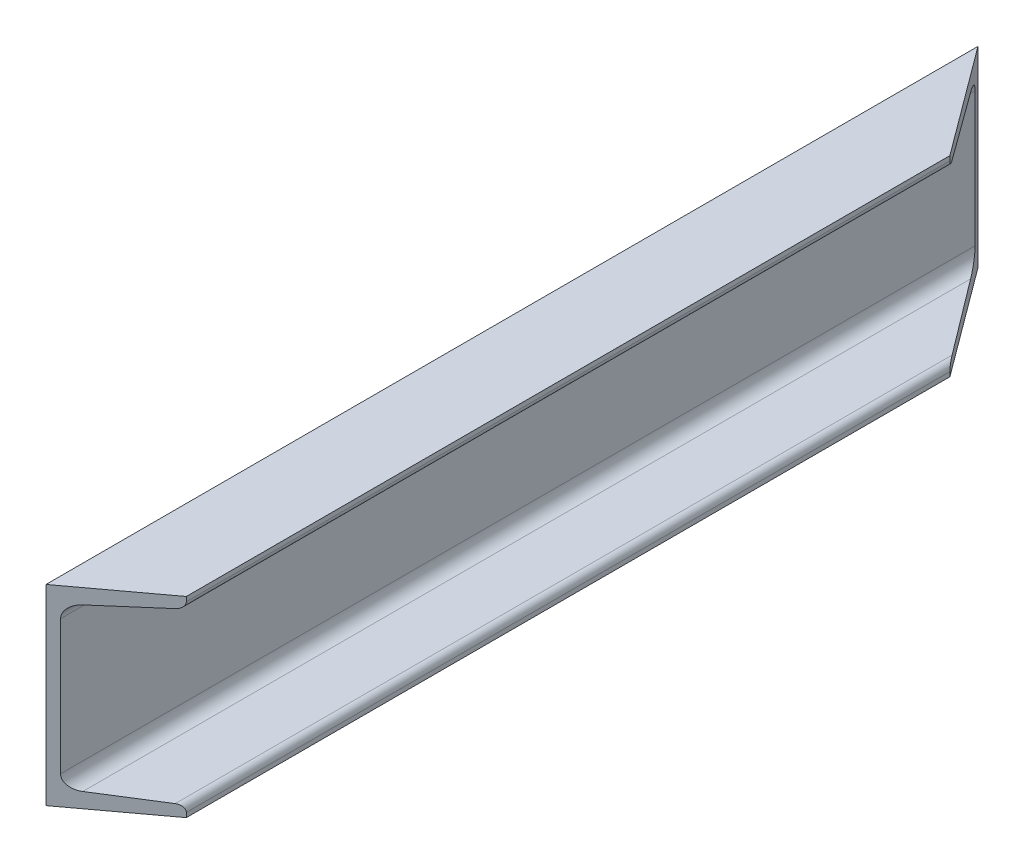
SolidWorks part; units mm, degrees
material "普通碳钢"
ref_plane "Front Plane" through (0, 0, 0) normal (0, 0, 1) x (1, 0, 0)
ref_plane "Top Plane" through (0, 0, 0) normal (0, 1, 0) x (1, 0, 0)
ref_plane "Right Plane" through (0, 0, 0) normal (1, 0, 0) x (0, 0, -1)
sketch "Sketch1" plane through (0, 0, 0) normal (0, 0, 1) x (1, 0, 0)
  line L0 (0, 63) -> (0, -63)
  line L1 (-28.7334, 0) -> (89.5233, 0) construction
  line L2 (0, 63) -> (53, 63)
  line L3 (53, 63) -> (53, 60.0159)
  line L4 (48.8069, 55.5264) -> (13.8863, 53.1396)
  line L5 (5.5, 44.1606) -> (5.5, -44.1606)
  line L6 (0, -63) -> (53, -63)
  line L7 (53, -63) -> (53, -60.0159)
  line L8 (48.8069, -55.5264) -> (13.8863, -53.1396)
  arc A0 (53, 60.0159) -> (48.8069, 55.5264) centre (48.5, 60.0159) cw
  arc A1 (13.8863, 53.1396) -> (5.5, 44.1606) centre (14.5, 44.1606) ccw
  arc A2 (13.8863, -53.1396) -> (5.5, -44.1606) centre (14.5, -44.1606) cw
  arc A3 (53, -60.0159) -> (48.8069, -55.5264) centre (48.5, -60.0159) ccw
  point P11 (53, 55.813)
  point P20 (53, -55.813)
  dimension "D5" = 4.5
  dimension "D6" = 9
  dimension "D9" = 9
  dimension "D10" = 4.5
  dimension "D1" = 126
  dimension "D2" = 7.187
  dimension "D3" = 3.91
  dimension "D4" = 5.5
  dimension "D7" = 7.187
  dimension "D8" = 3.91
  dimension "D11" = 53
  dimension "D12" = 53
extrude "Boss-Extrude1" add sketch "Sketch1" along normal mid plane 613
sketch "Sketch2" plane through (0, 63, 0) normal (0, 1, 0) x (1, 0, 0)
  line L0 (0, -306.5) -> (53, -267.2104)
  line L1 (53, -306.5) -> (53, 306.5) construction
  line L2 (53, -267.2104) -> (53, -306.5)
  line L3 (53, -306.5) -> (0, -306.5)
  line L4 (0, 306.5) -> (53, 235.0052)
  line L5 (53, 235.0052) -> (53, 306.5)
  line L6 (53, 306.5) -> (0, 306.5)
  dimension "D1" = 36.55
  dimension "D2" = 53.45
extrude "Cut-Extrude1" cut sketch "Sketch2" against normal blind 613
